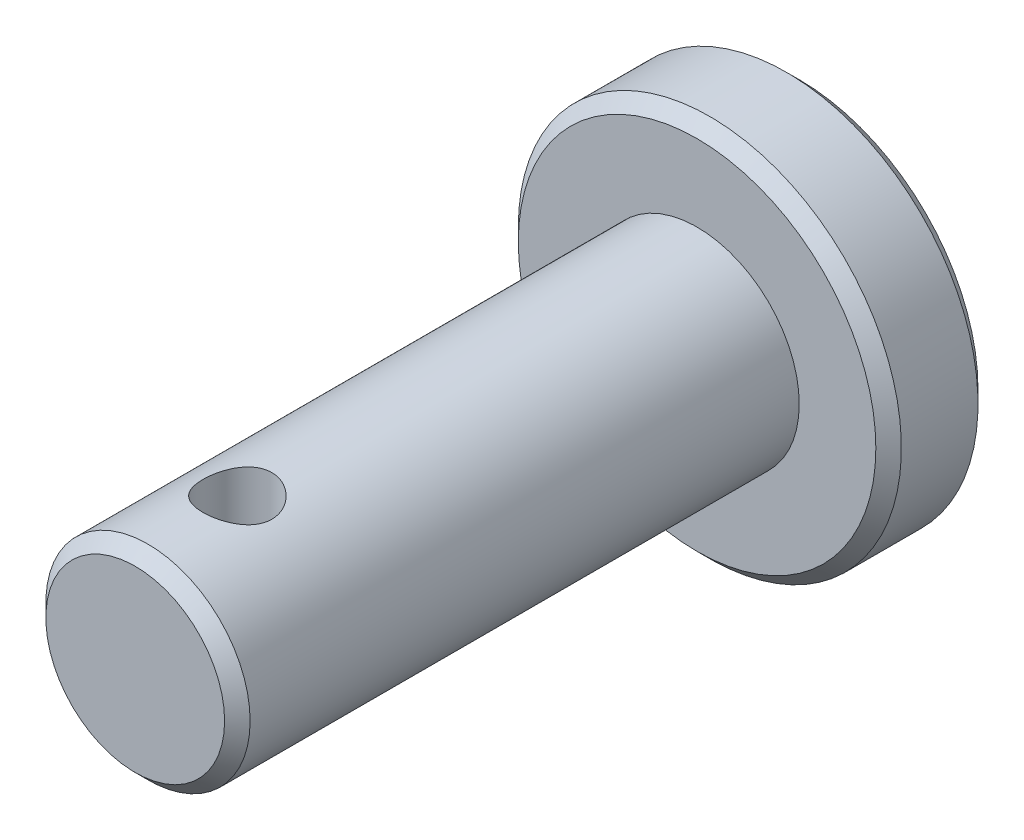
from build123d import *

# Parameters (mm, degrees)
SKETCH1_R               = 4
BOSS_EXTRUDE1_DEPTH     = 22
SKETCH2_R               = 7.5
BOSS_EXTRUDE2_DEPTH     = 4
CUT_EXTRUDE1_DEPTH      = 25.423349484
CUT_EXTRUDE1_DEPTH_BACK = 25.423349484
SKETCH3_R               = 1.35
CHAMFER1_SIZE           = 0.5


with BuildPart() as part:
    # Sketch1 → Boss-Extrude1 (new body)
    with BuildSketch(Plane.XY):
        Circle(SKETCH1_R)
    extrude(amount=BOSS_EXTRUDE1_DEPTH)

    # Sketch2 → Boss-Extrude2 (add)
    with BuildSketch(Plane(origin=(0, 0, 0), x_dir=(-1, 0, 0), z_dir=(0, 0, -1))):
        Circle(SKETCH2_R)
    extrude(amount=BOSS_EXTRUDE2_DEPTH)

    # Sketch3 → Cut-Extrude1 (cut, two sides: drawn at the far end of the back side and taken through both)
    with BuildSketch(Plane(origin=(0, 0, 0), x_dir=(1, 0, 0), z_dir=(0, 1, 0)).offset(-CUT_EXTRUDE1_DEPTH_BACK)):
        with Locations(Location((0, -18, 0), (0, 0, 270))):
            Circle(SKETCH3_R)
    extrude(amount=CUT_EXTRUDE1_DEPTH + CUT_EXTRUDE1_DEPTH_BACK, mode=Mode.SUBTRACT)

    # Chamfer1
    chamfer1_edges = [part.edges().sort_by_distance(p)[0] for p in [
        (-4, 0, 22),
        (7.5, 0, 0),
        (7.5, 0, -4),
    ]]
    chamfer(chamfer1_edges, length=CHAMFER1_SIZE)


solid = part.part
